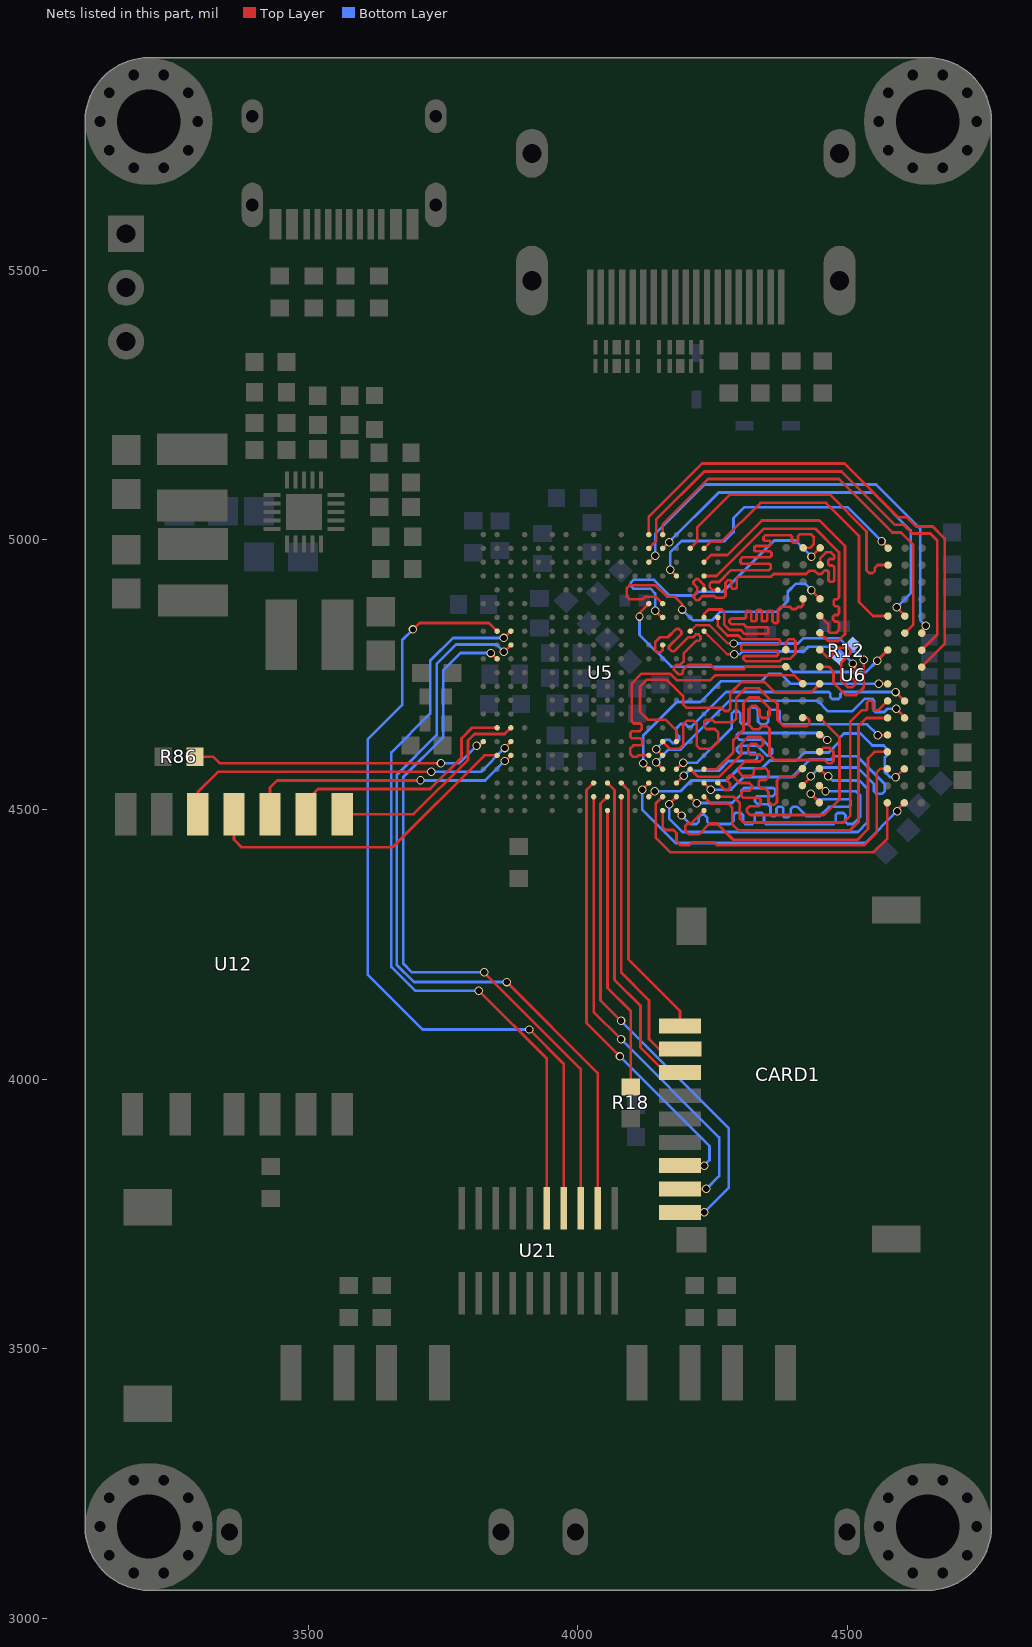
[diagram p0: the nets of this part, all layers, seen from the top]
# Altium PCB MISC105417.pcbdoc (part 4 of 5)
Units mil, origin at the board's own origin, x right, y up, seen from the top; angles counter-clockwise.
Board outline 1681.1 x 2842.52 mil, 4 copper layers (Top Layer, GND, PWR, Bottom Layer), stack 62.447 mil thick; 102 components, 152 nets, 737 pads, 611 vias.

## Via types
v1: diameter 15.7, hole 11.8, Top Layer to Bottom Layer, 611 vias

## Nets (pads, with @x,y where several pads share a name; then routed paths per layer and width w, separated by ;. In a path a pad name is that pad's centre, name@x,y a point inside that pad or via, vN(x,y) a via of type N, cw(c..) or ccw(c..) an arc to the next point about the centre after c; other vN are vias at no path point) (continued)
SA8: U5.V17 U6.T8 | length 535
  Top Layer w5: U5.V17@4259.52,4907.54 4249.28,4907.54 4244.47,4912.35 4244.47,4918.5 4247.91,4921.94 4262.12,4921.94 4284.2,4944.02 4354.55,4944.02 4357.5,4946.96 4357.5,4953.48 4355.14,4955.84 4303.77,4955.84 4301.53,4958.08 4301.53,4963.86 4305.35,4967.68 4355.84,4967.68 4359.07,4970.91 4359.07,4976.26 4356.39,4978.94 4328.88,4978.94 4327.62,4980.2 4327.62,4987.17 4329.39,4988.94 4354.77,4988.94 4357.2,4991.37 4357.2,4996.47 4355.03,4998.65 4346.2,4998.65 4344.2,5000.65 4344.2,5004.94 4348.2,5008.94 4394.5,5008.94 4397.2,5006.24 4397.2,4996.94 4399.2,4994.94 4405.2,4994.94 4408.2,4997.94 4408.2,5007.03 4411.78,5010.61 4432.17,5010.61 4437.18,5005.6 4437.18,4991.92 4430.65,4985.39 U6.T8@4417.84,4985.39
SA9: U5.T20 U6.R3 | length 535
  Top Layer w5: U5.T20@4208.34,4984.31 4221.2,4997.17 4221.2,5022.94 4282.2,5083.94 4467.2,5083.94 4535.2,5015.94 4535.2,4943.65 4540.2,4938.65 4546.59,4938.65 4550.76,4942.82 4550.76,4948.1 4556.05,4953.39 U6.R3@4575.24,4953.39
SA10: U5.U19 U6.L7 | length 535
  Top Layer w5: U5.U19@4233.93,4958.72 4247.15,4971.94 4277.2,4971.94 4341.2,5035.94 4448.2,5035.94 4495.46,4988.69 4495.46,4825.16 4482.61,4812.32 4464.32,4812.32 U6.L7@4448.84,4827.79
SA11: U5.U17 U6.R7 | length 535
  Top Layer w5: U5.U17@4233.93,4907.54 4233.93,4916.22 4222.46,4927.69 4219.23,4927.69 4214.23,4922.69 4214.23,4919.05 4221.2,4912.08 4221.2,4903.94 4214.2,4896.94 4214.2,4893.94 4220.2,4887.94 4223.2,4887.94 4231.49,4896.23 4252.76,4896.23 4256.05,4892.94 4270.57,4892.94 4273.75,4896.12 4273.75,4920.49 4278.69,4925.43 4283.33,4925.43 4284.53,4924.22 4284.53,4912.2 4287.19,4909.55 4292.25,4909.55 4294.81,4912.11 4294.81,4929.02 4297.74,4931.94 4358.29,4931.94 4363.29,4936.94 4423.27,4936.94 4429.27,4942.94 4439.2,4942.94 4445.2,4936.94 4451.32,4936.94 4457.77,4943.39 4462.58,4943.39 4464.86,4941.11 4464.86,4925.23 4467.71,4922.39 4473.03,4922.39 4475.2,4924.56 4475.2,4949.68 4472.29,4952.59 4466.94,4952.59 4464.2,4955.32 4464.2,4961.8 4467.13,4964.73 4473.46,4964.73 4475.2,4966.47 4475.2,4971.45 4469.71,4976.94 4460.2,4976.94 4449.24,4965.98 U6.R7@4449.24,4953.79
SA12: U5.P16 U6.N7 | length 535
  Top Layer w5: U5.P16@4157.16,4881.95 4144.17,4894.94 4125.2,4894.94 4120.2,4889.94 4095.73,4889.94 4090.73,4894.94 4090.73,4910.94 4095.73,4915.94 4144.2,4915.94 4165.2,4894.94 4179.09,4894.94 4193.2,4880.83 v1(4193.2,4870.94) ; v1(4433.2,4906.94) 4433.2,4906.63 U6.N7@4449.04,4890.79
  Bottom Layer w5: v1(4193.2,4870.94) 4213.2,4850.94 4248.2,4850.94 4263.92,4866.66 4368.92,4866.66 4389.2,4886.94 4389.2,4903.94 4404.2,4918.94 4421.2,4918.94 v1(4433.2,4906.94)
SA13: U5.R18 U6.T3 | length 535
  Top Layer w5: v1(4171.2,4944.94) 4171.2,4944.68 U5.R18@4182.75,4933.13 ; v1(4563.2,4997.94) 4563.2,4997.03 U6.T3@4575.34,4984.89
  Bottom Layer w5: v1(4171.2,4944.94) 4171.2,4976.94 4192.2,4997.94 4272.2,4997.94 4288.75,5014.49 4288.75,5040.91 4308.79,5060.94 4500.2,5060.94 v1(4563.2,4997.94)
SA14: U5.P15 U6.T7 | length 535
  Top Layer w5: v1(4143.2,4868.94) 4155.79,4856.36 U5.P15@4157.16,4856.36 ; v1(4433.2,4968.94) 4433.2,4969.16 U6.T7@4449.34,4985.29
  Bottom Layer w5: v1(4143.2,4868.94) 4143.2,4900.65 4134.23,4909.62 4103.04,4909.62 4098.15,4914.51 4098.15,4921.18 4102.91,4925.94 4141.2,4925.94 4170.12,4897.03 4215.62,4897.03 4222.54,4903.94 4269.2,4903.94 4364.2,4998.94 4403.2,4998.94 v1(4433.2,4968.94)
SA15: U5.U18 U6.M7 | length 535
  Top Layer w5: U5.U18@4233.93,4933.13 4257.1,4933.13 4344.91,5020.94 4440.2,5020.94 4484.2,4976.94 4484.2,4893.65 4480.5,4889.94 4476.67,4889.94 4474.67,4887.94 4474.67,4879.68 4477.41,4876.94 4482,4876.94 4484.2,4874.74 4484.2,4863.45 4481.7,4860.94 4476.08,4860.94 4473.08,4857.94 4473.08,4852.27 4476.53,4848.82 4481.39,4848.82 4484.2,4846 4484.2,4832.94 4479.2,4827.94 4467.2,4827.94 4464.2,4830.94 4464.2,4844.03 U6.M7@4448.94,4859.29
SBA0: U5.P20 U6.M2 | length 708.2
  Top Layer w5: U5.P20@4157.16,4984.31 4168.79,4995.94 v1(4169.2,4995.94) ; v1(4591.2,4874.94) 4606.44,4859.71 U6.M2@4606.44,4858.79
  Bottom Layer w5: v1(4169.2,4995.94) 4261.2,5087.94 4547.2,5087.94 4617.2,5017.94 4617.2,4900.94 v1(4591.2,4874.94)
SBA1: U5.U15 U6.N8 | length 535
  Top Layer w5: U5.U15@4233.93,4856.36 4233.93,4862.31 4242.5,4870.88 4266.89,4870.88 4271.2,4866.56 4271.2,4842.94 4281.2,4832.94 4302.2,4832.94 4309.2,4825.94 4352.2,4825.94 4353.2,4826.94 4353.2,4835.94 4351.2,4837.94 4313.2,4837.94 4307.2,4843.94 4284.2,4843.94 4281.24,4846.91 4281.24,4851.47 4284.08,4854.31 4309.66,4854.31 4311.85,4856.51 4311.85,4866.71 4313.96,4868.81 4319.55,4868.81 4321.46,4866.9 4321.46,4850.6 4322.94,4849.13 4329.54,4849.13 4331.39,4850.97 4331.39,4867.79 4333.54,4869.94 4339.11,4869.94 4341.02,4868.03 4341.02,4851.08 4342.86,4849.25 4348.95,4849.25 4350.92,4851.22 4350.92,4866.5 4353.36,4868.94 4358.84,4868.94 4361.08,4866.7 4361.08,4848.59 4363.53,4846.13 4368.77,4846.13 4371.19,4848.55 4371.19,4870.97 4376.38,4876.16 4392.9,4876.16 4397.16,4871.89 4404.23,4871.89 4408.02,4875.68 4414,4875.68 4417.54,4879.22 U6.N8@4417.54,4890.89
SBA2: U5.U20 U6.M3 | length 535
  Top Layer w5: U5.U20@4233.93,4984.31 4246.56,4996.94 4266.5,4996.94 4338.5,5068.94 4460.2,5068.94 4521.39,5007.76 4521.39,4885.01 4547.51,4858.89 U6.M3@4574.94,4858.89
SCAS: U5.N16 U6.K3 | length 571.5
  Top Layer w5: v1(4114.2,4857.94) 4114.2,4864.58 U5.N16@4131.57,4881.95 ; v1(4555.2,4775.94) 4555.2,4776.36 U6.K3@4574.74,4795.89
  Bottom Layer w5: v1(4114.2,4857.94) 4114.2,4823.94 4173.2,4764.94 4389.2,4764.94 4399.2,4754.94 4534.2,4754.94 v1(4555.2,4775.94)
SCKE0: U5.V15 U6.K9 | length 535
  Top Layer w5: U5.V15@4259.52,4856.36 4259.52,4840.54 4277.12,4822.94 4297.38,4822.94 4304.38,4815.94 4372.65,4815.94 4375,4813.59 4375,4808.9 4372.04,4805.94 4305.47,4805.94 4302.76,4803.23 4302.76,4796.76 4304.8,4794.72 4368.55,4794.72 4371,4792.28 4371,4787.22 4368.63,4784.85 4308.75,4784.85 4307.16,4783.26 4307.16,4779.33 4311.55,4774.94 4373.65,4774.94 4378.65,4779.94 4393.91,4779.94 4403.74,4789.77 4403.74,4812.04 4399.83,4815.94 4391.92,4815.94 4385.74,4809.76 U6.K9@4385.74,4796.49
SCKE1: U5.P13 U6.J9 | length 535
  Top Layer w5: U5.P13@4157.16,4805.18 4157.16,4795.9 4153.2,4791.94 4146.2,4791.94 4143.18,4794.96 4143.18,4810.29 4152.49,4819.59 4166.68,4819.59 4181.97,4834.89 4187.2,4834.89 4192.2,4829.89 4192.2,4825.94 4169.1,4802.84 4169.1,4798.34 4174.1,4793.34 4178.6,4793.34 4204.53,4819.27 4213.53,4819.27 4219.18,4824.91 4223.52,4824.91 4227.5,4820.94 4227.5,4816.01 4224.43,4812.94 4219.38,4812.94 4196.2,4789.77 4196.2,4774.53 4189.62,4767.94 4181.95,4767.94 4178.33,4764.32 4178.33,4758.81 4186.2,4750.94 4192.2,4750.94 4194.2,4752.94 4194.2,4757.94 4204.2,4767.94 4246.22,4767.94 4254.24,4759.92 4307.07,4759.92 4312.14,4764.99 U6.J9@4385.64,4764.99
SCKN: R12.1 U5.U14 U6.K7 | length 535
  Top Layer w4: U5.U14@4233.93,4830.77 4276.76,4787.94 v1(4290.2,4787.94)
  Top Layer w5: U6.K7@4448.74,4796.29 4462.09,4782.94 4468.2,4782.94 4473.2,4787.94 4473.2,4794.94 4478.2,4799.94 4501.2,4799.94 4505,4796.15 4505,4789.07 4488.2,4772.28 4488.2,4739.56 4501.06,4726.7 4508.77,4726.7 4514.2,4732.13 4514.2,4739.25 4511.59,4741.86 4508.43,4741.86 4506.04,4744.26 4506.04,4751.94 4508.04,4753.94 4511.42,4753.94 4514.2,4756.73 4514.2,4766.45 v1(4509.85,4770.8)
  Bottom Layer w5: v1(4290.2,4787.94) 4300.05,4787.94 4305.22,4793.1 4418.37,4793.1 4427.2,4801.94 4478.71,4801.94 v1(4509.85,4770.8)
SCKP: R12.2 U5.T14 U6.J7 | length 535
  Top Layer w4: U5.T14@4208.34,4830.77 4219.51,4841.94 4244.2,4841.94 4278.2,4807.94 v1(4289.2,4807.94)
  Top Layer w5: U6.J7@4448.64,4764.79 4465.35,4764.79 4474.2,4755.94 4474.2,4734.74 4496.74,4712.21 4515.85,4712.21 4530.2,4726.56 v1(4530.2,4777.94)
  Bottom Layer w5: v1(4289.2,4807.94) 4408.2,4807.94 4418.2,4817.94 4484.2,4817.94 4509.45,4792.7 4516.52,4792.7 4530.2,4779.01 v1(4530.2,4777.94)
SCS0: U5.P21 U6.L2 | length 739.5
  Top Layer w5: U5.P21@4157.16,5009.91 4157.16,5028.7 4241.4,5112.94 4484.2,5112.94 4583.2,5013.94 4599.2,5013.94 4622.2,4990.94 4622.2,4843.16 U6.L2@4606.34,4827.29
SCS1: U5.N19 U6.L1 | length 822.2
  Top Layer w5: U5.N19@4131.57,4958.72 4143.2,4970.35 v1(4143.2,4970.94) ; U6.L1@4637.84,4827.19 4637.84,4833.58 v1(4645.2,4840.94)
  Bottom Layer w5: v1(4143.2,4970.94) 4143.2,5011.24 4234.91,5102.94 4553.2,5102.94 4634.85,5021.29 4634.85,4851.94 4645.2,4841.59 v1(4645.2,4840.94)
SDC0_CLK: R18.1 U5.K1 | length 530.3
  Top Layer w5: U5.K1@4054.8,4498.09 4054.8,4169.2 4098,4126 R18.1@4098,3985.66
SDC0_CMD: CARD1.3 U5.K3 | length 608.3
  Top Layer w5: U5.K3@4054.8,4549.28 4068,4536.08 4068,4184 4116,4136 4116,4059 4162.6,4012.4 CARD1.3@4189.4,4012.4
SDC0_D0: CARD1.7 U5.J3 | length 858.4
  Top Layer w5: U5.J3@4029.2,4549.28 4016,4536.08 4016,4104 v1(4078,4042) ; CARD1.7@4189.4,3839.5 v1(4234,3839.5)
  Bottom Layer w5: v1(4078,4042) 4244,3876 4244,3849.5 v1(4234,3839.5)
SDC0_D1: CARD1.8 U5.J2 | length 882.4
  Top Layer w5: U5.J2@4029.2,4523.69 4029.2,4124.8 v1(4080,4074) ; CARD1.8@4189.4,3796.3 v1(4238,3796.3)
  Bottom Layer w5: v1(4080,4074) 4262,3892 4262,3820.3 v1(4238,3796.3)
SDC0_D2: CARD1.1 U5.L3 | length 495.7
  Top Layer w5: U5.L3@4080.39,4549.28 4094,4535.67 4094,4222 4189.4,4126.6 CARD1.1@4189.4,4098.7
SDC0_D3: CARD1.2 U5.L2 | length 536.2
  Top Layer w5: U5.L2@4080.39,4523.69 4080.39,4197.61 4132,4146 4132,4074 4150.4,4055.6 CARD1.2@4189.5,4055.6
SDC0_DET: CARD1.9 U5.K2 | length 938.4
  Top Layer w5: U5.K2@4054.8,4523.69 4042,4510.89 4042,4146 v1(4080,4108) ; CARD1.9@4189.4,3752.8 v1(4234,3752.8)
  Bottom Layer w5: v1(4080,4108) 4280,3908 4280,3798.8 v1(4234,3752.8)
SDC1_CLK: R86.2 U5.A6 | length 556.4
  Top Layer w5: R86.2@3289.66,4598 3323.48,4598 3335.48,4586 v1(3746,4586) ; v1(3812,4618) 3816.43,4618 U5.A6@3824.48,4626.05
  Bottom Layer w5: v1(3746,4586) 3780,4586 v1(3812,4618)
SDC1_CMD: U5.C7 U12.1 | length 400.4
  Top Layer w5: U12.1@3562.72,4491.33 3695.33,4491.33 3796,4592 3796,4628 3808,4640 3864.02,4640 U5.C7@3875.66,4651.64
SDC1_D0: U5.C6 U12.5 | length 661.1
  Top Layer w5: U12.5@3295.01,4491.33 3295.01,4533.01 3332,4570 v1(3728,4570) ; v1(3864,4614) 3864,4614.39 U5.C6@3875.66,4626.05
  Bottom Layer w5: v1(3728,4570) 3820,4570 v1(3864,4614)
SDC1_D1: U5.B5 U12.4 | length 611.8
  Top Layer w5: U12.4@3361.94,4491.33 3361.94,4444.06 3376,4430 3656,4430 3826.46,4600.46 U5.B5@3850.07,4600.46
SDC1_D2: U5.C5 U12.3 | length 521
  Top Layer w5: U12.3@3428.87,4491.33 3428.87,4540.87 3442,4554 v1(3708,4554) ; v1(3864,4590) 3865.2,4590 U5.C5@3875.66,4600.46
  Bottom Layer w5: v1(3708,4554) 3828,4554 v1(3864,4590)
SDC1_D3: U5.B7 U12.2 | length 456.1
  Top Layer w5: U12.2@3495.8,4491.33 3495.8,4515.8 3518,4538 3726,4538 3784,4596 3784,4632 3803.64,4651.64 U5.B7@3850.07,4651.64
SDQ0: U5.N3 U6.A2 | length 598.4
  Top Layer w5: v1(4119.2,4536.94) U5.N3@4131.57,4549.28 ; v1(4592.2,4496.94) 4592.2,4499.16 U6.A2@4605.34,4512.29
  Bottom Layer w5: v1(4119.2,4536.94) 4119.2,4499.94 4181.2,4437.94 4533.2,4437.94 v1(4592.2,4496.94)
SDQ1: U5.U4 U6.D7 | length 598.4
  Top Layer w5: U5.U4@4233.93,4574.87 4256.79,4574.87 4288.2,4606.28 4288.2,4629.14 4307,4647.94 4307,4697.73 4317.2,4707.94 4335.2,4707.94 4355.2,4687.94 4355.2,4674.94 4350.2,4669.94 4341.67,4669.94 4336.67,4674.94 4336.67,4685.48 4330.2,4691.94 4323.2,4691.94 4317.22,4685.96 4317.22,4656.39 4324.68,4648.93 4335.65,4648.93 4341.66,4654.94 4350.2,4654.94 4355.2,4649.94 4355.2,4600.94 4364.2,4591.94 4457.2,4591.94 4463.2,4585.94 4470.2,4585.94 4474.2,4589.94 4474.2,4606.94 4466.54,4614.61 4455.45,4614.61 U6.D7@4448.14,4607.29
SDQ2: U5.N2 U6.C2 | length 598.4
  Top Layer w5: U5.N2@4131.57,4523.69 4141.82,4533.94 v1(4142.2,4533.94) ; v1(4589.2,4559.94) 4604.56,4575.29 U6.C2@4605.54,4575.29
  Bottom Layer w5: v1(4142.2,4533.94) 4190.2,4533.94 4210.2,4553.94 4275.72,4553.94 4298.35,4576.57 4341.41,4576.57 4355.78,4590.94 4405.2,4590.94 4420.2,4605.94 4465.28,4605.94 4485.2,4625.87 4485.2,4632.94 4493.2,4640.94 4523.9,4640.94 4546.03,4618.82 4567.03,4618.82 4574.12,4611.73 4574.12,4601.63 4569.12,4596.63 4569.12,4569.49 4578.67,4559.94 v1(4589.2,4559.94)
SDQ3: U5.T4 U6.C8 | length 598.4
  Top Layer w5: U5.T4@4208.34,4574.87 4222.27,4560.94 4262.2,4560.94 4302.34,4601.08 4302.34,4621.7 4315.24,4634.6 4338.19,4634.6 4343.19,4629.6 4343.19,4620.94 4339.19,4616.94 4335.2,4616.94 4330.2,4621.94 4321,4621.94 4316,4616.94 4316,4605.95 4319.79,4602.16 4337.2,4602.16 4342.2,4597.16 4342.2,4593.39 4337.92,4589.1 4309.85,4589.1 4298.38,4577.64 4298.38,4569.19 4305.42,4562.15 4321.13,4562.15 4326.2,4567.23 4326.2,4572.89 4330.15,4576.83 4347.71,4576.83 4353.65,4570.89 4353.65,4560.51 4348.08,4554.94 4338.2,4554.94 4335.2,4551.94 4335.2,4543.94 4340.2,4538.94 4347.2,4538.94 4353.65,4532.5 4353.65,4514.5 4359.2,4508.94 4364.46,4508.94 4369.2,4513.69 4369.2,4553.97 4376.17,4560.94 4401.59,4560.94 U6.C8@4416.54,4575.89
SDQ4: U5.U3 U6.B8 | length 598.4
  Top Layer w5: U5.U3@4233.93,4549.22 v1(4246.2,4536.94) ; U6.B8@4416.44,4544.39 4432.2,4560.16 v1(4432.2,4561.94)
  Bottom Layer w5: v1(4246.2,4536.94) 4284.2,4536.94 4307.59,4560.33 4397.48,4560.33 4430.09,4592.94 4469.2,4592.94 4475.2,4598.94 4517.2,4598.94 4569.22,4546.92 4569.22,4534.06 4564.22,4529.06 4554.04,4529.06 4549.04,4534.06 4549.04,4547.52 4518.62,4577.94 4448.2,4577.94 v1(4432.2,4561.94)
SDQ5: U5.P1 U6.C3 | length 598.4
  Top Layer w5: U5.P1@4157.16,4498.09 4157.16,4467.5 4162.72,4461.94 4177.07,4461.94 4182.79,4456.22 4182.79,4441.36 4190.2,4433.94 4206.47,4433.94 4211.47,4438.94 4252.71,4438.94 4257.71,4433.94 4531.2,4433.94 4554.2,4456.94 4554.2,4568.94 4560.66,4575.39 U6.C3@4574.04,4575.39
SDQ6: U5.T2 U6.A7 | length 598.4
  Top Layer w5: U5.T2@4208.34,4523.69 4220.09,4511.94 v1(4220.2,4511.94) ; v1(4432.2,4528.94) 4447.84,4513.31 U6.A7@4447.84,4512.79
  Bottom Layer w5: v1(4220.2,4511.94) 4286.17,4511.94 4303.2,4528.98 4303.2,4534.94 4308.2,4539.94 4362.45,4539.94 4366.14,4536.26 4366.14,4529.42 4361.14,4524.42 4332.35,4524.42 4328.5,4520.57 4328.5,4515.06 4333.77,4509.79 4352.3,4509.79 4357.2,4504.88 4357.2,4490.94 4360.2,4487.94 4365.66,4487.94 4368.2,4490.49 4368.2,4501.94 4371.57,4505.31 4377.58,4505.31 4381.11,4501.78 4381.11,4487.94 4383.11,4485.94 4390.2,4485.94 4394.91,4490.65 4394.91,4500.94 4399.28,4505.31 4406.2,4505.31 4423.92,4487.58 4448.17,4487.58 4465.46,4504.87 4501.49,4504.87 4505.52,4508.91 4505.52,4516.63 4502.96,4519.19 4441.96,4519.19 v1(4432.2,4528.94)
SDQ7: U5.P2 U6.A3 | length 598.4
  Top Layer w5: U5.P2@4157.16,4523.69 4144.2,4510.73 4144.2,4447.94 4171.2,4420.94 4548.2,4420.94 4573.84,4446.57 U6.A3@4573.84,4512.39
SDQ8: U5.P5 U6.G2 | length 575.4
  Top Layer w5: v1(4145.2,4611.94) 4145.68,4611.94 U5.P5@4157.16,4600.46 ; v1(4589.2,4717.94) U6.G2@4605.94,4701.29
  Bottom Layer w5: v1(4145.2,4611.94) 4162.61,4629.35 4169.8,4629.35 4175.61,4623.53 4182.89,4623.53 4187.49,4628.14 4187.49,4635.65 4182.37,4640.78 4182.37,4650.6 4190.55,4658.78 4199.37,4658.78 4204.33,4653.81 4210.74,4653.81 4274.87,4717.94 4465.05,4717.94 4468.2,4714.79 4468.2,4708.33 4471.5,4705.04 4483.38,4705.04 4487.2,4708.86 4487.2,4714.69 4490.46,4717.94 v1(4589.2,4717.94)
SDQ9: U5.V3 U6.F7 | length 575.4
  Top Layer w5: U5.V3@4259.52,4549.28 4272.86,4535.94 4279.2,4535.94 4282.2,4538.94 4282.2,4547.94 4277.2,4552.94 4277.2,4558.94 4281.2,4562.94 4286.2,4562.94 4299.87,4549.28 4317.87,4549.28 4323.2,4543.94 4323.2,4539.69 4318.45,4534.94 4306.66,4534.94 4302.99,4531.28 4302.99,4525.37 4306.46,4521.9 4334.98,4521.9 4338.49,4518.39 4338.49,4509.23 4335.17,4505.9 4318.03,4505.9 4313.2,4501.07 4313.2,4495.94 4319.2,4489.94 4456.2,4489.94 4485.2,4518.94 4485.2,4633.43 U6.F7@4448.34,4670.29
SDQ10: U5.P4 U6.F2 | length 575.4
  Top Layer w5: v1@4144.9,4587.44 4157.16,4575.18 U5.P4@4157.16,4574.87 ; v1(4590.2,4686.94) 4605.84,4671.31 U6.F2@4605.84,4669.79
  Bottom Layer w5: v1(4144.9,4587.47) 4168.37,4610.94 4190.2,4610.94 4281.2,4701.94 4444.2,4701.94 4464.04,4682.11 4508.73,4682.11 4531.86,4705.23 4546.27,4705.23 4549.2,4702.3 4549.2,4683.38 4551.65,4680.94 4568.2,4680.94 4574.2,4686.94 v1(4590.2,4686.94)
SDQ11: U5.R4 U6.E3 | length 575.4
  Top Layer w5: U5.R4@4182.75,4574.87 4194.82,4586.94 v1(4195.2,4586.94) ; v1(4556.2,4637.94) 4573.79,4637.94 U6.E3@4574.24,4638.39
  Bottom Layer w5: v1(4195.2,4586.94) 4221.2,4586.94 4285.34,4651.08 4285.34,4678.16 4290.1,4682.92 4296.44,4682.92 4301.2,4678.16 4301.2,4661.64 4304.9,4657.94 4312.2,4657.94 4317.2,4662.94 4317.2,4685.94 4320.2,4688.94 4329.2,4688.94 4334.2,4683.94 4334.2,4662.94 4339.2,4657.94 4347.46,4657.94 4353.2,4663.69 4353.2,4680.94 4357.2,4684.94 4371.2,4684.94 4374.2,4681.94 4374.2,4663.46 4379.72,4657.94 4536.2,4657.94 v1(4556.2,4637.94)
SDQ12: U5.R6 U6.H7 | length 575.4
  Top Layer w5: U5.R6@4182.75,4626.05 4182.75,4646.4 4162.36,4666.79 4129.55,4666.79 4115.23,4681.11 4115.23,4728.34 4127.4,4740.5 4165.65,4740.5 4195.2,4710.94 4195.2,4694.78 4201.04,4688.94 4266.23,4688.94 4272.37,4682.81 4278.72,4682.81 4282.56,4686.64 4282.56,4715.7 4303.42,4736.56 4345.78,4736.56 4365.4,4716.94 4432.19,4716.94 U6.H7@4448.54,4733.29
SDQ13: U5.N4 U6.H3 | length 575.4
  Top Layer w5: v1(4121.2,4585.94) 4121.2,4585.24 U5.N4@4131.57,4574.87 ; v1(4558.1,4733.43) 4574,4733.43 U6.H3@4574.54,4732.89
  Bottom Layer w5: v1(4121.2,4585.94) 4121.2,4637.24 4183.36,4699.39 4226.98,4699.39 4265.53,4737.94 4340.71,4737.94 4354.71,4751.94 4375.93,4751.94 4394.44,4733.43 v1(4558.1,4733.43)
SDQ14: U5.P6 U6.F8 | length 575.4
  Top Layer w5: U5.P6@4157.16,4626.05 4170.27,4612.94 4188.2,4612.94 4195.2,4619.94 4195.2,4657.94 4202.2,4664.94 4214.2,4664.94 4220.2,4658.94 4220.2,4618.51 4225.77,4612.94 4247.2,4612.94 4260.45,4626.19 4260.45,4642.69 4253.85,4649.29 4238.26,4649.29 4234.2,4653.35 4234.2,4662.94 4237.2,4665.94 4249.52,4665.94 4253.52,4661.94 4286.6,4661.94 4293.83,4669.18 4293.83,4707.57 4311.2,4724.94 4335.2,4724.94 4357.25,4702.89 4363.25,4702.89 4370.2,4695.94 4370.2,4666.32 4381.58,4654.94 4424.92,4654.94 4429.01,4659.03 4429.01,4666.23 4424.84,4670.39 U6.F8@4416.84,4670.39
SDQ15: U5.N5 U6.H8 | length 575.4
  Top Layer w5: U5.N5@4131.57,4600.46 4111.99,4600.46 4109.34,4597.81 4101.87,4597.81 4097.09,4602.59 4097.09,4612.88 4103.15,4618.94 4116.2,4618.94 4119.2,4621.94 4119.2,4628.94 4116.2,4631.94 4100.15,4631.94 4097.5,4634.6 4097.5,4642.49 4099.95,4644.94 4114.2,4644.94 4118.2,4648.94 4118.2,4656.94 4115.6,4659.55 4103.3,4659.55 4099.91,4662.94 4099.91,4733.65 4118.19,4751.93 4171.22,4751.93 4183.24,4739.91 4245.64,4739.91 4254.67,4748.94 4401.49,4748.94 U6.H8@4417.04,4733.39
SDQM0: U5.U1 U6.D3 | length 598.4
  Top Layer w5: U5.U1@4233.93,4498.09 4209.78,4473.94 4203.2,4473.94 4199.2,4469.94 4199.2,4460.58 4205.85,4453.94 4224.2,4453.94 4244.2,4473.94 4258.08,4473.94 4288.08,4443.94 4518.2,4443.94 4538.2,4463.94 4538.2,4594.94 4550.16,4606.89 U6.D3@4574.14,4606.89
SDQM1: U5.R3 U6.E7 | length 575.4
  Top Layer w5: U5.R3@4182.75,4549.28 4182.75,4549.49 v1(4196.2,4562.94) ; U6.E7@4448.24,4638.79 4458.09,4628.94 v1(4462.2,4628.94)
  Bottom Layer w5: v1(4196.2,4562.94) 4205.2,4571.94 4261.2,4571.94 4279.14,4589.88 4327.53,4589.88 4332.53,4594.88 4332.53,4600.94 4328.53,4604.94 4298.8,4604.94 4295.17,4608.57 4295.17,4614.26 4299.09,4618.17 4333.1,4618.17 4350.92,4600.36 4356.28,4600.36 4360.15,4604.23 4360.15,4611.66 4342.32,4629.49 4299.43,4629.49 4294.98,4633.94 4294.98,4638.94 4297.98,4641.94 4449.2,4641.94 v1(4462.2,4628.94)
SDQS0N: U5.R1 U6.B7 | length 598.4
  Top Layer w5: U5.R1@4182.75,4498.09 4191.9,4488.94 v1(4192.2,4488.94) ; U6.B7@4447.94,4544.29 4448.85,4544.29 v1(4459.2,4533.94)
  Bottom Layer w5: v1(4192.2,4488.94) 4207.97,4473.18 4219.77,4473.18 4224.2,4477.61 4224.2,4485.99 4228.87,4490.65 4233.95,4490.65 4239.78,4484.82 4239.78,4478.06 4244.67,4473.18 4282.94,4473.18 4289.2,4479.44 4289.2,4490.94 4292.2,4493.94 4302.2,4493.94 4306.2,4489.94 4306.2,4477.43 4310.45,4473.18 4323.41,4473.18 4328.17,4477.94 ; 4328.2,4477.94 4328.2,4490.94 4331.2,4493.94 4341.2,4493.94 4345.2,4489.94 4345.2,4476.65 4348.68,4473.18 4474.46,4473.18 ; v1(4459.2,4533.94) 4516.16,4533.94 4523.11,4526.99 4523.11,4486.39 4509.9,4473.18 4500.19,4473.18 4496.37,4477 4496.37,4489.79 4492.49,4493.67 4481.98,4493.67 4478.09,4489.78 4478.09,4476.73 4474.46,4473.1
SDQS0P: U5.R2 U6.C7 | length 598.4
  Top Layer w5: v1(4169.2,4509.94) 4169.2,4510.14 U5.R2@4182.75,4523.69 ; U6.C7@4448.04,4575.79 4461.89,4561.94 v1(4464.2,4561.94)
  Bottom Layer w5: v1(4169.2,4509.94) 4169.2,4482.94 4193.83,4458.32 4519.21,4458.32 4536.48,4475.59 4536.48,4539.48 4522.02,4553.94 4472.2,4553.94 v1(4464.2,4561.94)
SDQS1N: U5.V2 U6.G3 | length 575.4
  Top Layer w5: U5.V2@4259.52,4523.69 4288.46,4523.69 4300.2,4511.94 4300.2,4482.94 4307.05,4476.09 4492.14,4476.09 4505.33,4489.28 4505.33,4663.06 4526.2,4683.94 4533.9,4683.94 4536.2,4686.24 4536.2,4698.43 4539.32,4701.55 4544.37,4701.55 4547.2,4698.72 4547.2,4686.94 4550.2,4683.94 4556.99,4683.94 U6.G3@4574.44,4701.39
SDQS1P: U5.U2 U6.F3 | length 575.4
  Top Layer w5: U5.U2@4233.93,4523.69 4246.68,4510.94 4279.2,4510.94 4286.2,4503.94 4286.2,4472.94 4298.2,4460.94 4504.26,4460.94 4520.46,4477.14 4520.46,4655.16 4535.19,4669.89 U6.F3@4574.34,4669.89
SODT0: U5.N20 U6.K1 | length 885.6
  Top Layer w5: U5.N20@4131.57,4984.31 4145.2,4997.94 4145.2,5037.79 4234.36,5126.94 4489.2,5126.94 4588.2,5027.94 4604.2,5027.94 4620.2,5011.94 4653.5,5011.94 4666.55,4998.89 4666.55,4824.51 U6.K1@4637.74,4795.69
SODT1: U5.N21 U6.J1 | length 937
  Top Layer w5: U5.N21@4131.57,5009.91 4131.57,5043.49 4230.02,5141.94 4494.2,5141.94 4594.2,5041.94 4610.2,5041.94 4627.2,5024.94 4658.2,5024.94 4680.2,5002.94 4680.2,4806.76 U6.J1@4637.64,4764.19
SPI1_CLK: U5.C14 U21.15 | length 1406.1
  Top Layer w5: v1(3816,4164) 3942.19,4037.81 U21.15@3942.19,3760.55 ; v1(3862.2,4818.27) 3863.16,4818.27 U5.C14@3875.66,4830.77
  Bottom Layer w5: v1(3816,4164) 3698,4164 3654,4208 3654,4606 3726,4678 3726,4776 3768.27,4818.27 v1(3862.2,4818.27)
SPI1_CS: U5.B14 U21.14 | length 1542.2
  Top Layer w5: v1(3694,4834) 3706,4846 3834.84,4846 U5.B14@3850.07,4830.77 ; v1(3910,4092) 3973.68,4028.32 U21.14@3973.68,3760.55
  Bottom Layer w5: v1(3694,4834) 3674,4814 3674,4694 3610,4630 3610,4194 3712,4092 v1(3910,4092)
SPI1_MISO: U5.C13 U21.12 | length 1458.3
  Top Layer w5: v1(3862.2,4792.94) 3863.42,4792.94 U5.C13@3875.66,4805.18 ; v1(3868,4180) 4036.68,4011.32 U21.12@4036.68,3760.55
  Bottom Layer w5: v1(3862.2,4792.94) 3849.15,4806 3774,4806 3738,4770 3738,4638 3664,4564 3664,4212 3696,4180 v1(3868,4180)
SPI1_MOSI: U5.B12 U21.13 | length 1360.8
  Top Layer w5: v1(3826,4198) 4005.18,4018.82 U21.13@4005.18,3760.55 ; v1(3838.2,4790.28) 3839.38,4790.28 U5.B12@3850.07,4779.59
  Bottom Layer w5: v1(3826,4198) 3692,4198 3676,4214 3676,4560 3750,4634 3750,4758 3782.28,4790.28 v1(3838.2,4790.28)